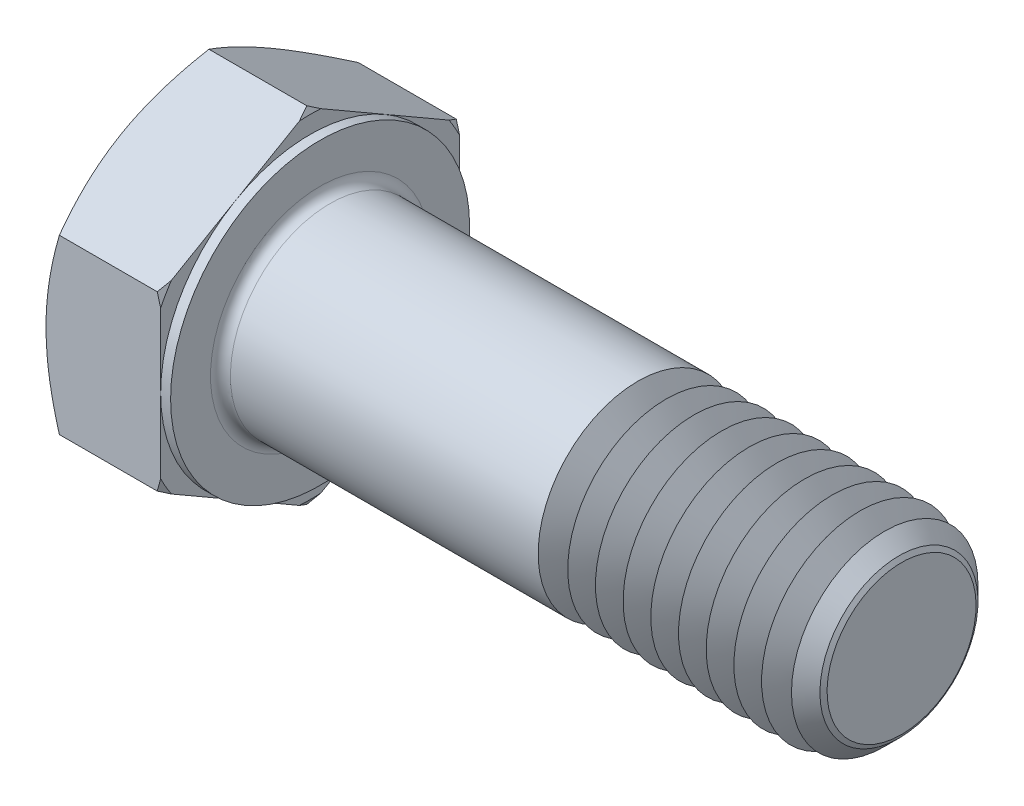
from build123d import *

# Parameters (mm, degrees)
EXTRUDE_364_DEPTH      = 7.5
SKETCH_4_W             = 0.6
SKETCH_4_H             = 11.392304845
CHAMFER_2049_SIZE      = 1.4
FILLET_2094_R          = 0.6
PATTERN_LINEAR_1_COUNT = 10
PATTERN_LINEAR_1_PITCH = 1.666666667


with BuildPart() as part:
    # 草图1 → Extrude 364 (new body)
    with BuildSketch(Plane(origin=(0, 0, 0), x_dir=(0, 0, -1), z_dir=(1, 0, 0))):
        Polygon((9, 5.196152423), (9, -5.196152423), (0, -10.392304845), (-9, -5.196152423), (-9, 5.196152423), (0, 10.392304845), align=None)
    extrude(amount=EXTRUDE_364_DEPTH)

    # 草图2 → 凸台-旋转1 (revolve)
    with BuildSketch(Plane.XY, mode=Mode.PRIVATE) as revolve_1_sk:
        Polygon((0, 0), (42.5, 0), (42.5, 4.4845), (42.5, 6), (7.791693541, 6), (0, 6), align=None)
    revolve(revolve_1_sk.sketch.rotate(Axis((0, 0, 0), (1, 0, 0)), 90), axis=Axis((0, 0, 0), (1, 0, 0)))

    # 草图3 → 切除-旋转1 (revolve, cut)
    with BuildSketch(Plane.XY):
        Polygon((0, 9), (3.690598923, 15.392304845), (3.690598923, 20.392304845), (-10, 20.392304845), (-10, 9), align=None)
    revolve(axis=Axis((0, 0, 0), (1, 0, 0)), mode=Mode.SUBTRACT)

    # 草图5 → 切除-旋转2 (revolve, cut)
    with BuildSketch(Plane.XY):
        Polygon((7.5, 9), (3.809401077, 15.392304845), (3.809401077, 20.392304845), (13.809401077, 20.392304845), (13.809401077, 9), align=None)
    revolve(axis=Axis((0, 0, 0), (1, 0, 0)), mode=Mode.SUBTRACT)

    # 草图4 → 切除-旋转3 (revolve, cut)
    with BuildSketch(Plane.XY, mode=Mode.PRIVATE) as cut_revolve_3_sk:
        with Locations((7.2, 14.696152423)):
            Rectangle(SKETCH_4_W, SKETCH_4_H)
    revolve(cut_revolve_3_sk.sketch.rotate(Axis((0, 0, 0), (1, 0, 0)), 270), axis=Axis((0, 0, 0), (1, 0, 0)), mode=Mode.SUBTRACT)

    # Chamfer 2049
    chamfer_2049_edges = [part.edges().sort_by_distance(p)[0] for p in [
        (42.5, 0, -6),
    ]]
    chamfer(chamfer_2049_edges, length=CHAMFER_2049_SIZE)

    # Fillet 2094
    fillet_2094_edges = [part.edges().sort_by_distance(p)[0] for p in [
        (7.5, 0, -6),
    ]]
    fillet(fillet_2094_edges, radius=FILLET_2094_R)

    # 草图6 → 切除-旋转4 (revolve, cut)
    with BuildSketch(Plane.XY):
        Polygon((27.5, -4.4845), (26.625025667, -6), (26.625025667, -7.5), (28.374974333, -7.5), (28.374974333, -6), align=None)
    cut_revolve_4 = revolve(axis=Axis((-3.175, 0, 0), (1, 0, 0)), mode=Mode.SUBTRACT)

    # 阵列(线性)1: 切除-旋转4 ×10
    with Locations(*[(i * PATTERN_LINEAR_1_PITCH, 0, 0) for i in range(1, PATTERN_LINEAR_1_COUNT)]):
        add(cut_revolve_4, mode=Mode.SUBTRACT)


solid = part.part
